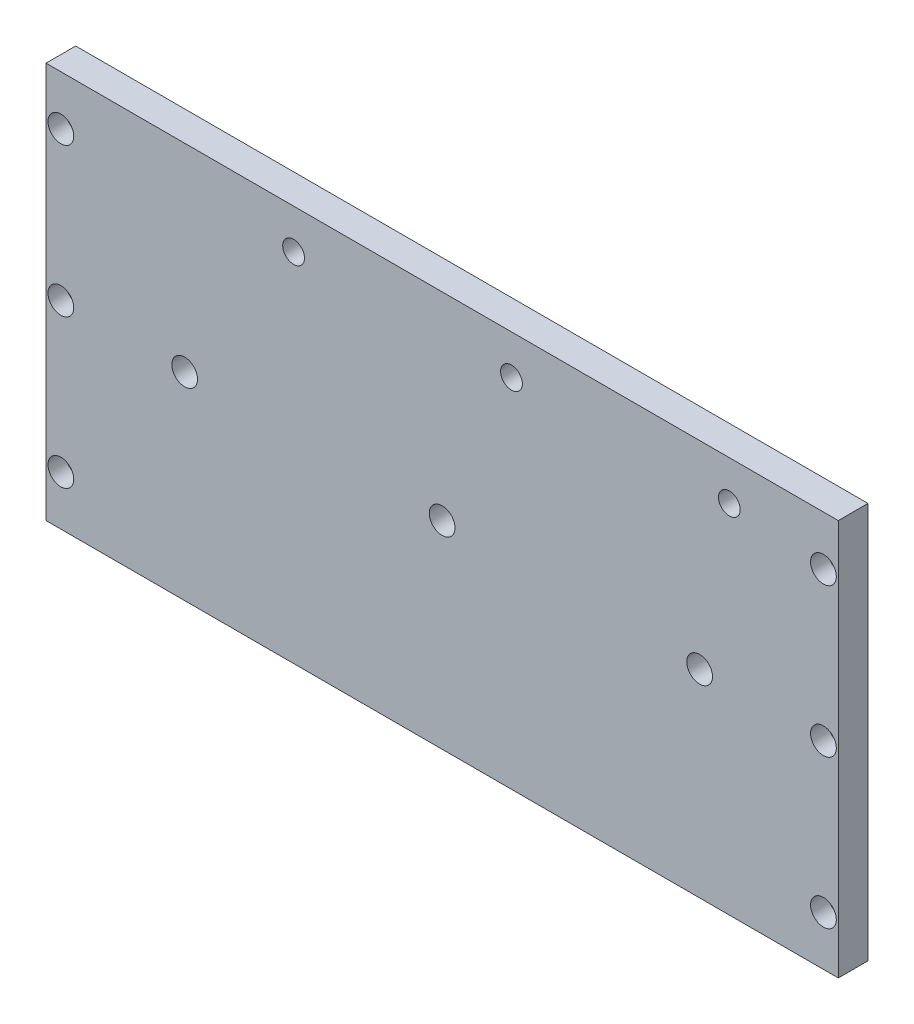
from build123d import *

# Parameters (mm, degrees)
SKETCH1_W               = 400
SKETCH1_H               = 200
BOSS_EXTRUDE1_DEPTH     = 15
SKETCH2_R               = 6.5
CUT_EXTRUDE1_DEPTH      = 9
LPATTERN1_COUNT         = 3
LPATTERN1_PITCH         = 75
MIRROR1_COPY_1_SKETCH_R = 6.5
MIRROR1_COPY_1_DEPTH    = 9
MIRROR1_COPY_2_SKETCH_R = 6.5
MIRROR1_COPY_2_DEPTH    = 9
SKETCH3_R               = 4.5
CUT_EXTRUDE2_DEPTH      = 85
LPATTERN2_COUNT         = 3
LPATTERN2_PITCH         = 75
MIRROR2_COPY_1_SKETCH_R = 4.5
MIRROR2_COPY_1_DEPTH    = 85
MIRROR2_COPY_2_SKETCH_R = 4.5
MIRROR2_COPY_2_DEPTH    = 85
SKETCH4_R               = 6.5
CUT_EXTRUDE3_DEPTH      = 85
LPATTERN3_COUNT         = 3
LPATTERN3_PITCH         = 130
SKETCH5_R               = 5.5
CUT_EXTRUDE4_DEPTH      = 51
LPATTERN4_COUNT         = 3
LPATTERN4_PITCH         = 110


with BuildPart() as part:
    # Sketch1 → Boss-Extrude1 (new body)
    with BuildSketch(Plane.XY):
        Rectangle(SKETCH1_W, SKETCH1_H)
    extrude(amount=BOSS_EXTRUDE1_DEPTH)

    # Sketch2 → Cut-Extrude1 (cut)
    with BuildSketch(Plane.XY.offset(15)):
        with Locations((-192.5, 75)):
            Circle(SKETCH2_R)
    cut_extrude1 = extrude(amount=-CUT_EXTRUDE1_DEPTH, mode=Mode.SUBTRACT)

    # LPattern1: Cut-Extrude1 ×3
    with Locations(*[(0, -i * LPATTERN1_PITCH, 0) for i in range(1, LPATTERN1_COUNT)]):
        add(cut_extrude1, mode=Mode.SUBTRACT)

    # Mirror1: Cut-Extrude1 across plane
    add(cut_extrude1.mirror(Plane(origin=(0, 0, 0), x_dir=(0, 0, 1), z_dir=(1, 0, 0))), mode=Mode.SUBTRACT)

    # Mirror1 copy 1 sketch → Mirror1 copy 1 (cut)
    with BuildSketch(Plane(origin=(0, -75, 15), x_dir=(-1, 0, 0), z_dir=(0, 0, 1))):
        with Locations((-192.5, -75)):
            Circle(MIRROR1_COPY_1_SKETCH_R)
    extrude(amount=-MIRROR1_COPY_1_DEPTH, mode=Mode.SUBTRACT)

    # Mirror1 copy 2 sketch → Mirror1 copy 2 (cut)
    with BuildSketch(Plane(origin=(0, -150, 15), x_dir=(-1, 0, 0), z_dir=(0, 0, 1))):
        with Locations((-192.5, -75)):
            Circle(MIRROR1_COPY_2_SKETCH_R)
    extrude(amount=-MIRROR1_COPY_2_DEPTH, mode=Mode.SUBTRACT)

    # Sketch3 → Cut-Extrude2 (cut)
    with BuildSketch(Plane.XY.offset(15)):
        with Locations((-192.5, 75)):
            Circle(SKETCH3_R)
    cut_extrude2 = extrude(amount=-CUT_EXTRUDE2_DEPTH, mode=Mode.SUBTRACT)

    # LPattern2: Cut-Extrude2 ×3
    with Locations(*[(0, -i * LPATTERN2_PITCH, 0) for i in range(1, LPATTERN2_COUNT)]):
        add(cut_extrude2, mode=Mode.SUBTRACT)

    # Mirror2: Cut-Extrude2 across plane
    add(cut_extrude2.mirror(Plane(origin=(0, 0, 0), x_dir=(0, 0, 1), z_dir=(1, 0, 0))), mode=Mode.SUBTRACT)

    # Mirror2 copy 1 sketch → Mirror2 copy 1 (cut)
    with BuildSketch(Plane(origin=(0, -75, 15), x_dir=(-1, 0, 0), z_dir=(0, 0, 1))):
        with Locations((-192.5, -75)):
            Circle(MIRROR2_COPY_1_SKETCH_R)
    extrude(amount=-MIRROR2_COPY_1_DEPTH, mode=Mode.SUBTRACT)

    # Mirror2 copy 2 sketch → Mirror2 copy 2 (cut)
    with BuildSketch(Plane(origin=(0, -150, 15), x_dir=(-1, 0, 0), z_dir=(0, 0, 1))):
        with Locations((-192.5, -75)):
            Circle(MIRROR2_COPY_2_SKETCH_R)
    extrude(amount=-MIRROR2_COPY_2_DEPTH, mode=Mode.SUBTRACT)

    # Sketch4 → Cut-Extrude3 (cut)
    with BuildSketch(Plane.XY.offset(15)):
        with Locations((-130, 0)):
            Circle(SKETCH4_R)
    cut_extrude3 = extrude(amount=-CUT_EXTRUDE3_DEPTH, mode=Mode.SUBTRACT)

    # LPattern3: Cut-Extrude3 ×3
    with Locations(*[(i * LPATTERN3_PITCH, 0, 0) for i in range(1, LPATTERN3_COUNT)]):
        add(cut_extrude3, mode=Mode.SUBTRACT)

    # Sketch5 → Cut-Extrude4 (cut)
    with BuildSketch(Plane.XY.offset(15)):
        with Locations((-75, 80)):
            Circle(SKETCH5_R)
    cut_extrude4 = extrude(amount=-CUT_EXTRUDE4_DEPTH, mode=Mode.SUBTRACT)

    # LPattern4: Cut-Extrude4 ×3
    with Locations(*[(i * LPATTERN4_PITCH, 0, 0) for i in range(1, LPATTERN4_COUNT)]):
        add(cut_extrude4, mode=Mode.SUBTRACT)


solid = part.part
